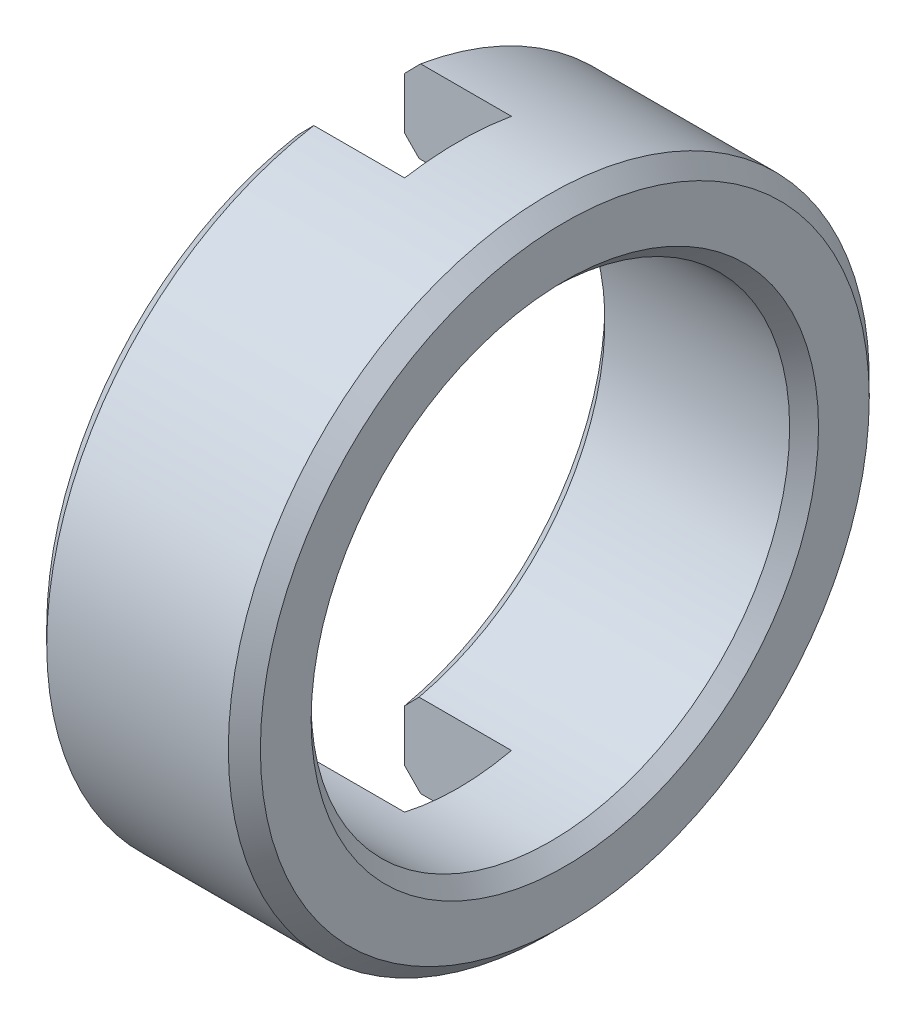
from build123d import *

# Parameters (mm, degrees)
CUT_EXTRUDE1_DEPTH      = 1
CUT_EXTRUDE1_DEPTH_BACK = 1
SKETCH2_W               = 5
SKETCH2_H               = 20


with BuildPart() as part:
    # Sketch1 → Revolve1 (revolve)
    with BuildSketch(Plane.XY, mode=Mode.PRIVATE) as revolve1_sk:
        Polygon((-2, 5.7), (-2, 4.75), (-1.7295, 4.4795), (1.7295, 4.4795), (2, 4.75), (2, 5.7), (1.7, 6), (-1.7, 6), align=None)
    revolve(revolve1_sk.sketch.rotate(Axis((2, 0, 0), (-1, 0, 0)), 270), axis=Axis((2, 0, 0), (-1, 0, 0)))

    # Sketch2 → Cut-Extrude1 (cut, two sides: drawn at the far end of the back side and taken through both)
    with BuildSketch(Plane.XY.offset(-CUT_EXTRUDE1_DEPTH_BACK)):
        with Locations((-2.5, 0)):
            Rectangle(SKETCH2_W, SKETCH2_H)
    extrude(amount=CUT_EXTRUDE1_DEPTH + CUT_EXTRUDE1_DEPTH_BACK, mode=Mode.SUBTRACT)


solid = part.part
